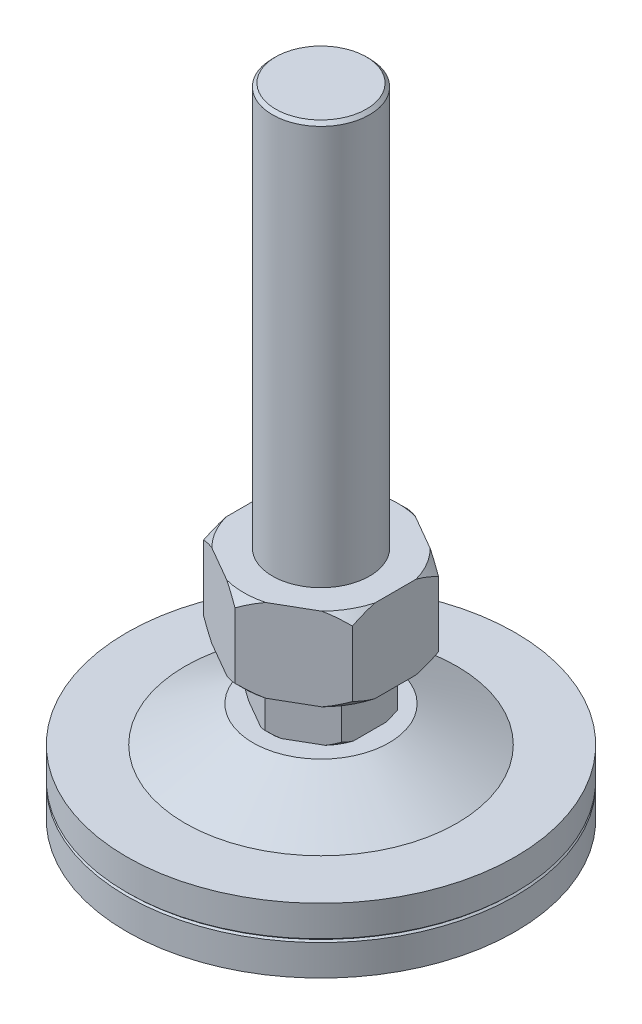
SolidWorks part; units mm, degrees
material "普通碳钢"
ref_plane "Front Plane" through (0, 0, 0) normal (0, 0, 1) x (1, 0, 0)
ref_plane "Top Plane" through (0, 0, 0) normal (0, 1, 0) x (1, 0, 0)
ref_plane "Right Plane" through (0, 0, 0) normal (1, 0, 0) x (0, 0, -1)
sketch "Sketch1" plane through (0, 0, 0) normal (0, 0, 1) x (1, 0, 0)
  line L0 (35, 0) -> (60, 0)
  line L1 (60, 0) -> (60, 9.5)
  line L2 (60, 20) -> (42, 20)
  line L3 (42, 20) -> (21, 31)
  line L4 (21, 31) -> (15, 31)
  line L5 (15, 31) -> (15, 197)
  line L6 (15, 197) -> (0, 197)
  line L7 (0, 197) -> (0, 15)
  line L8 (60, 10) -> (59.189, 10) construction
  line L9 (60, 10.5) -> (59.5, 10)
  line L10 (59.5, 10) -> (60, 9.5)
  line L11 (0, 15) -> (14, 15)
  line L12 (14, 15) -> (35, 0)
  line L13 (66, 0) -> (-66, 0) construction
  line L14 (60, 10.5) -> (60, 20)
  line L15 (0, 15) -> (0, 0) construction
  point P0 (7.5, 197)
  dimension "D1" = 20
  dimension "D2" = 197
  dimension "D3" = 15
  dimension "D4" = 6
  dimension "D5" = 31
  dimension "D6" = 18
  dimension "D7" = 60
  dimension "D8" = 10
  dimension "D9" = 0.5
  dimension "D10" = 1
  dimension "D11" = 0.5
  dimension "D12" = 15
  dimension "D13" = 25
  dimension "D14" = 14
  dimension "D15" = 45
revolve "Revolve1" add sketch "Sketch1" angle 360 about L7
cosmetic thread "Cosmetic Thread1" parameters "D2"=29
cosmetic thread "Cosmetic Thread2" parameters "D2"=29
sketch "Sketch2" plane through (0, 31, 0) normal (0, 1, 0) x (1, 0, 0)
  line L1 (15, 8.6603) -> (0, 17.3205)
  line L2 (0, 17.3205) -> (-15, 8.6603)
  line L3 (-15, 8.6603) -> (-15, -8.6603)
  line L4 (-15, -8.6603) -> (0, -17.3205)
  line L5 (0, -17.3205) -> (15, -8.6603)
  line L6 (15, -8.6603) -> (15, 8.6603)
  circle A0 centre (0, 0) radius 15 construction
  dimension "D1" = 30
extrude "Boss-Extrude1" add sketch "Sketch2" along normal blind 15
sketch "Sketch3" plane through (0, 0, 0) normal (1, 0, 0) x (0, 0, -1)
  line L0 (15.8205, 31) -> (17.3205, 32.5)
  line L1 (8.6603, 31) -> (17.3205, 31) construction
  line L2 (17.3205, 46) -> (17.3205, 31) construction
  line L3 (17.3205, 32.5) -> (17.3205, 31)
  line L4 (17.3205, 44.5) -> (15.8205, 46)
  line L5 (8.6603, 46) -> (12.9904, 46) construction
  line L6 (15.8205, 46) -> (17.3205, 46)
  line L7 (17.3205, 46) -> (17.3205, 44.5)
  line L8 (21, 31) -> (-21, 31) construction
  line L9 (17.3205, 31) -> (15.8205, 31)
  dimension "D1" = 45
  dimension "D2" = 1.5
  dimension "D3" = 45
  dimension "D4" = 1.5
revolve "Cut-Revolve1" cut sketch "Sketch3" angle 360 about axis through (0, 197, 0) along (0, 1, 0)
ref_plane "Plane1" through (0, 47, 0) normal (0, 1, 0) x (-1, 0, 0)
sketch "Sketch5" plane through (0, 47, 0) normal (0, 1, 0) x (-1, 0, 0)
  line L1 (0, 26.5581) -> (-23, 13.2791)
  line L2 (-23, 13.2791) -> (-23, -13.2791)
  line L3 (-23, -13.2791) -> (0, -26.5581)
  line L4 (0, -26.5581) -> (23, -13.2791)
  line L5 (23, -13.2791) -> (23, 13.2791)
  line L6 (23, 13.2791) -> (0, 26.5581)
  circle A0 centre (0, 0) radius 23 construction
  circle A1 centre (0, 0) radius 15
  dimension "D1" = 46
  dimension "D2" = 30
extrude "Boss-Extrude2" add sketch "Sketch5" along normal blind 25.6
sketch "Sketch7" plane through (0, 0, 0) normal (1, 0, 0) x (0, 0, -1)
  line L0 (23.8581, 72.6) -> (26.5581, 69.9)
  line L1 (13.2791, 72.6) -> (26.5581, 72.6) construction
  line L2 (26.5581, 72.6) -> (26.5581, 47) construction
  line L3 (26.5581, 69.9) -> (26.5581, 72.6)
  line L4 (26.5581, 72.6) -> (23.8581, 72.6)
  line L5 (23.8581, 47) -> (26.5581, 49.7)
  line L6 (23.1, 47) -> (-23.1, 47) construction
  line L7 (26.5581, 49.7) -> (26.5581, 47)
  line L8 (26.5581, 47) -> (23.8581, 47)
  dimension "D1" = 45
  dimension "D2" = 2.7
  dimension "D3" = 2.7
  dimension "D4" = 45
revolve "Cut-Revolve3" cut sketch "Sketch7" angle 360 about axis through (0, 197, 0) along (0, 1, 0)
chamfer "Chamfer1" distance 1 angle 45 1 edges at (-15, 197, 0)
